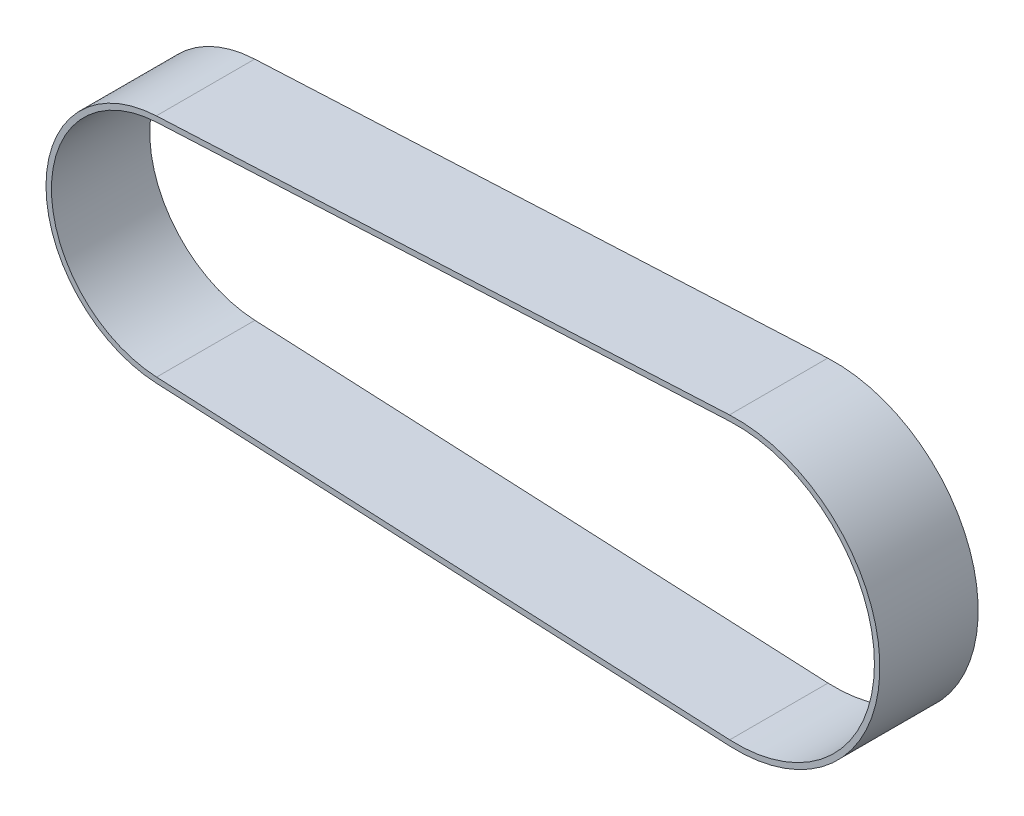
SolidWorks part; units mm, degrees
material "PE"
ref_plane "Front Plane" through (0, 0, 0) normal (0, 0, 1) x (1, 0, 0)
ref_plane "Top Plane" through (0, 0, 0) normal (0, 1, 0) x (1, 0, 0)
ref_plane "Right Plane" through (0, 0, 0) normal (1, 0, 0) x (0, 0, -1)
sketch "Sketch1" plane through (0, 0, 0) normal (0, 0, 1) x (1, 0, 0)
  line L0 (0, 0) -> (208, 0) construction
  line L1 (-1.9231, 39.9537) -> (205.5962, 49.9422)
  line L2 (-1.9231, -39.9537) -> (205.5962, -49.9422)
  line L3 (-2.0175, 41.9152) -> (205.5017, 51.9036)
  line L4 (-2.0175, -41.9152) -> (205.5017, -51.9036)
  arc A0 (-1.9231, 39.9537) -> (-1.9231, -39.9537) centre (0, 0) ccw
  arc A1 (205.5962, -49.9422) -> (205.5962, 49.9422) centre (208, 0) ccw
  arc A2 (205.5017, -51.9036) -> (205.5017, 51.9036) centre (208, 0) ccw
  arc A3 (-2.0175, 41.9152) -> (-2.0175, -41.9152) centre (0, 0) ccw
  point P14 (-2.0175, 41.9152)
  point P15 (-2.0175, -41.9152)
  point P16 (205.5017, 51.9036)
  point P17 (205.5017, -51.9036)
  dimension "D1" = 80
  dimension "D2" = 100
  dimension "D5" = 168.2472
  dimension "D4" = 127.7964
  dimension "D3" = 208
  dimension "D6" = 207.7595
extrude "Boss-Extrude1" add sketch "Sketch1" along normal blind 35.6
